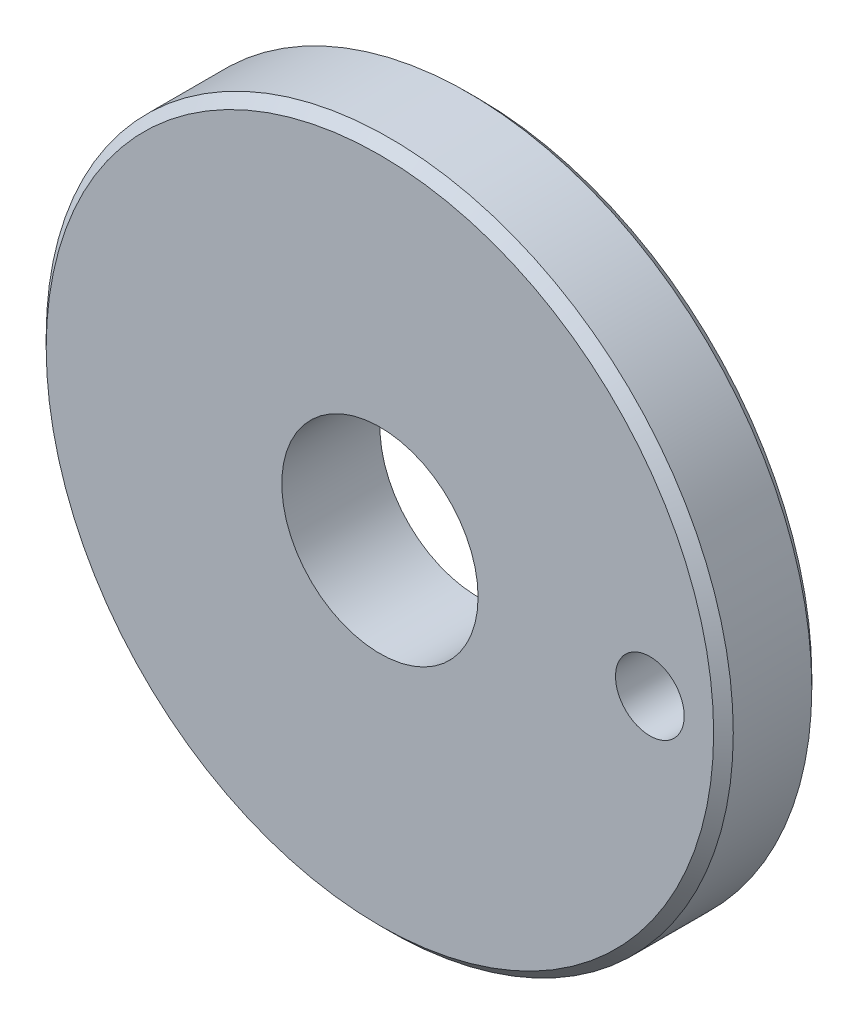
from build123d import *

# Parameters (mm, degrees)
SKETCH1_R           = 35
BOSS_EXTRUDE1_DEPTH = 10
CHAMFER1_SIZE       = 1
SKETCH2_R           = 10
CUT_EXTRUDE1_DEPTH  = 30
SKETCH3_R           = 3.5
CUT_EXTRUDE2_DEPTH  = 29


with BuildPart() as part:
    # Sketch1 → Boss-Extrude1 (new body)
    with BuildSketch(Plane.XY):
        Circle(SKETCH1_R)
    extrude(amount=BOSS_EXTRUDE1_DEPTH)

    # Chamfer1
    chamfer1_edges = [part.edges().sort_by_distance(p)[0] for p in [
        (-35, 0, 0),
        (-35, 0, 10),
    ]]
    chamfer(chamfer1_edges, length=CHAMFER1_SIZE)

    # Sketch2 → Cut-Extrude1 (cut)
    with BuildSketch(Plane.XY.offset(10)):
        Circle(SKETCH2_R)
    extrude(amount=-CUT_EXTRUDE1_DEPTH, mode=Mode.SUBTRACT)

    # Sketch3 → Cut-Extrude2 (cut)
    with BuildSketch(Plane.XY.offset(10)):
        with Locations((27.5, 0)):
            Circle(SKETCH3_R)
    extrude(amount=-CUT_EXTRUDE2_DEPTH, mode=Mode.SUBTRACT)


solid = part.part
